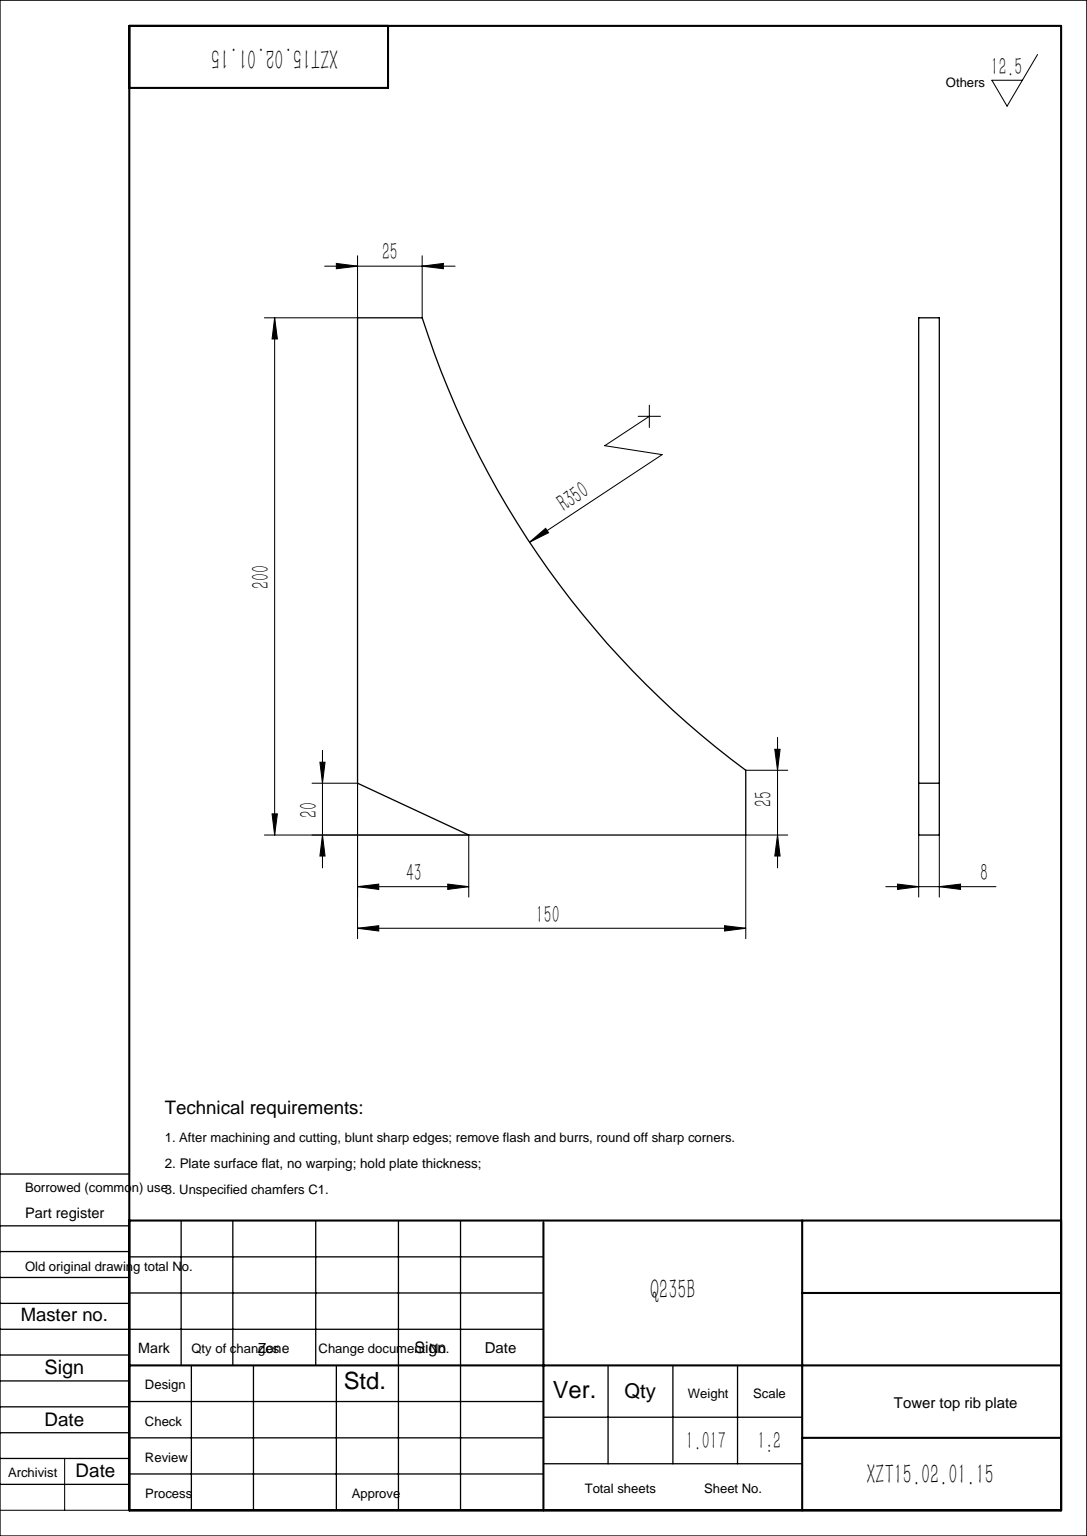
SolidWorks part; units mm, degrees
material "Q235B"
ref_plane "Front Plane" through (0, 0, 0) normal (0, 0, 1) x (1, 0, 0)
ref_plane "Top Plane" through (0, 0, 0) normal (0, 1, 0) x (1, 0, 0)
ref_plane "Right Plane" through (0, 0, 0) normal (1, 0, 0) x (0, 0, -1)
sketch "Sketch1" plane through (0, 0, 0) normal (0, 0, 1) x (1, 0, 0)
  line L0 (0, 0) -> (150, 0)
  line L1 (150, 0) -> (150, 25)
  line L2 (150, 25) -> (25, 200)
  line L3 (25, 200) -> (0, 200)
  line L4 (0, 200) -> (0, 0)
  dimension "D1" = 150
  dimension "D2" = 25
  dimension "D3" = 25
  dimension "D4" = 200
extrude "Boss-Extrude1" add sketch "Sketch1" along normal mid plane 8
chamfer "Chamfer1" distance 20 distance2 43 1 edges at (0, 0, 0)
sketch "Sketch2" plane through (0, 0, 4) normal (0, 0, 1) x (1, 0, 0)
  line L6 (0, 200) -> (0, 20)
  line L7 (0, 20) -> (43, 0)
  line L8 (43, 0) -> (150, 0)
  line L9 (150, 0) -> (150, 25)
  line L10 (150, 25) -> (25, 200)
  line L11 (25, 200) -> (0, 200)
  line L12 (0, 200) -> (0, 20)
  line L13 (0, 20) -> (43, 0)
  line L14 (43, 0) -> (150, 0)
  line L15 (150, 0) -> (150, 25)
  line L16 (150, 25) -> (25, 200)
  line L17 (25, 200) -> (0, 200)
  arc A0 (25, 200) -> (150, 25) centre (358.5325, 306.0946) ccw
  line M11 (150, 25) -> (25, 200)
  dimension "D1" = 350
  dimension "D2" = 0
extrude "Cut-Extrude1" cut sketch "Sketch2" against normal blind 10 contours A0 M11
